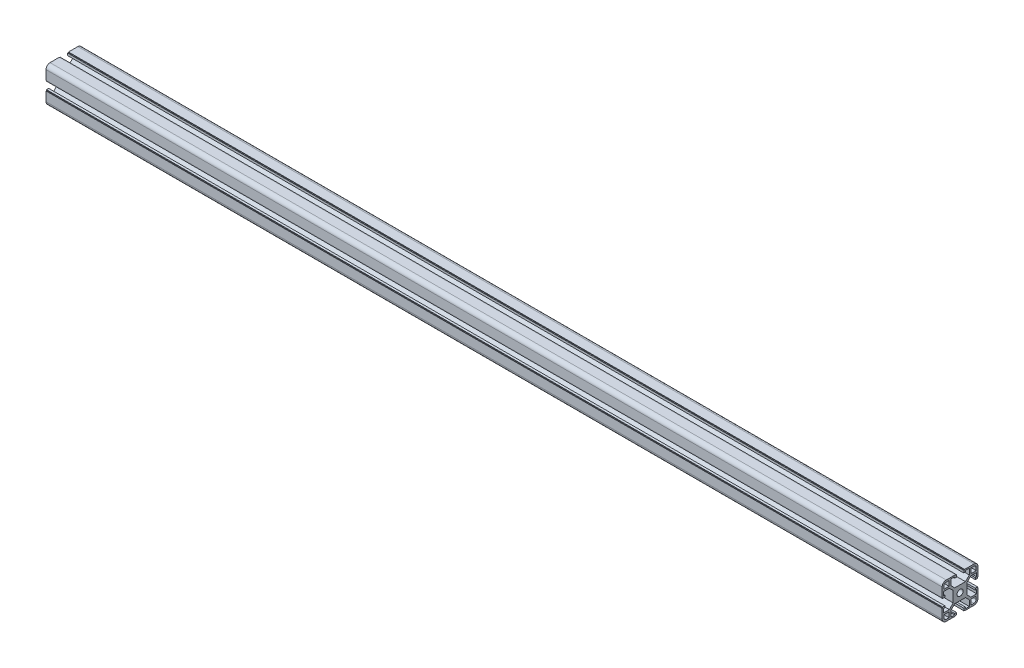
SolidWorks part; units mm, degrees
ref_plane "Front Plane" through (0, 0, 0) normal (0, 0, 1) x (1, 0, 0)
ref_plane "Top Plane" through (0, 0, 0) normal (0, 1, 0) x (1, 0, 0)
ref_plane "Right Plane" through (0, 0, 0) normal (1, 0, 0) x (0, 0, -1)
sketch "草图1" plane through (0, 0, 0) normal (0, 0, 1) x (1, 0, 0)
  line L0 (0, 0) -> (1000, 0)
  dimension "D1" = 1000
other "Aluminum profile 40 X 40B X R4.5(1)"
ref_plane "Plane1" through (0, 0, 0) normal (1, 0, 0) x (0, 1, 0)
sketch "Sketch1" plane through (0, 0, 0) normal (1, 0, 0) x (0, 1, 0)
  line L0 (-5.1, 20) -> (-5.1, 19.5)
  line L1 (-5.1, 19.5) -> (-4.1, 19.5)
  line L2 (-4.1, 19.5) -> (-4.1, 17)
  line L3 (-6.1, 18.5) -> (-10.3, 18.5)
  line L4 (-15.5, -20) -> (-5.1, -20)
  line L5 (-20, -15.5) -> (-20, -5.1)
  line L6 (15.5, 20) -> (5.1, 20)
  line L7 (20, 15.5) -> (20, 5.1)
  line L8 (0, 14.8756) -> (0, 0) construction
  line L9 (0, 0) -> (14.1675, 0) construction
  line L10 (-10.3, 18.5) -> (-10.3, 12)
  line L11 (-10.3, 12) -> (-6, 7.7)
  line L12 (-6, 7.7) -> (6, 7.7)
  line L13 (10.3, 12) -> (6, 7.7)
  line L14 (10.3, 18.5) -> (10.3, 12)
  line L15 (6.1, 18.5) -> (10.3, 18.5)
  line L16 (4.1, 19.5) -> (4.1, 17)
  line L17 (5.1, 19.5) -> (4.1, 19.5)
  line L18 (5.1, 20) -> (5.1, 19.5)
  line L19 (-5.1, 20) -> (-15.5, 20)
  line L20 (20, 5.1) -> (19.5, 5.1)
  line L21 (12.3, 18) -> (15.5, 18)
  line L22 (12.3, 18) -> (12.3, 12.3)
  line L23 (12.3, 12.3) -> (18, 12.3)
  line L24 (18, 15.5) -> (18, 12.3)
  line L25 (19.5, 5.1) -> (19.5, 4.1)
  line L26 (19.5, 4.1) -> (17, 4.1)
  line L27 (17, 6.1) -> (17, 4.1)
  line L28 (18.5, 6.1) -> (17, 6.1)
  line L29 (18.5, 6.1) -> (18.5, 10.3)
  line L30 (18.5, 10.3) -> (12, 10.3)
  line L31 (12, 10.3) -> (7.7, 6)
  line L32 (7.7, 6) -> (7.7, -6)
  line L33 (12, -10.3) -> (7.7, -6)
  line L34 (18.5, -10.3) -> (12, -10.3)
  line L35 (18.5, -6.1) -> (18.5, -10.3)
  line L36 (18.5, -6.1) -> (17, -6.1)
  line L37 (17, -4.1) -> (17, -6.1)
  line L38 (19.5, -4.1) -> (17, -4.1)
  line L39 (19.5, -5.1) -> (19.5, -4.1)
  line L40 (20, -5.1) -> (19.5, -5.1)
  line L41 (5.1, -20) -> (5.1, -19.5)
  line L42 (5.1, -19.5) -> (4.1, -19.5)
  line L43 (4.1, -19.5) -> (4.1, -17)
  line L44 (6.1, -17) -> (4.1, -17)
  line L45 (6.1, -18.5) -> (6.1, -17)
  line L46 (6.1, -18.5) -> (10.3, -18.5)
  line L47 (10.3, -18.5) -> (10.3, -12)
  line L48 (10.3, -12) -> (6, -7.7)
  line L49 (6, -7.7) -> (-6, -7.7)
  line L50 (-10.3, -12) -> (-6, -7.7)
  line L51 (-10.3, -18.5) -> (-10.3, -12)
  line L52 (-6.1, -18.5) -> (-10.3, -18.5)
  line L53 (-6.1, -18.5) -> (-6.1, -17)
  line L54 (-4.1, -17) -> (-6.1, -17)
  line L55 (-4.1, -19.5) -> (-4.1, -17)
  line L56 (-5.1, -19.5) -> (-4.1, -19.5)
  line L57 (-5.1, -20) -> (-5.1, -19.5)
  line L58 (-20, -5.1) -> (-19.5, -5.1)
  line L59 (5.1, -20) -> (15.5, -20)
  line L60 (-20, 5.1) -> (-20, 15.5)
  line L61 (-19.5, -5.1) -> (-19.5, -4.1)
  line L62 (-6.1, 18.5) -> (-6.1, 17)
  line L63 (-6.1, 17) -> (-4.1, 17)
  line L64 (6.1, 18.5) -> (6.1, 17)
  line L65 (4.1, 17) -> (6.1, 17)
  line L66 (-19.5, -4.1) -> (-17, -4.1)
  line L67 (-15.5, 18) -> (-12.3, 18)
  line L68 (-18, 15.5) -> (-18, 12.3)
  line L69 (-18, 12.3) -> (-12.3, 12.3)
  line L70 (-12.3, 18) -> (-12.3, 12.3)
  line L71 (-17, -6.1) -> (-17, -4.1)
  line L72 (-18.5, -6.1) -> (-17, -6.1)
  line L73 (-18.5, -6.1) -> (-18.5, -10.3)
  line L74 (-18.5, -10.3) -> (-12, -10.3)
  line L75 (-12, -10.3) -> (-7.7, -6)
  line L76 (-7.7, -6) -> (-7.7, 6)
  line L77 (-12, 10.3) -> (-7.7, 6)
  line L78 (-18.5, 10.3) -> (-12, 10.3)
  line L79 (-18.5, 6.1) -> (-18.5, 10.3)
  line L80 (-18.5, 6.1) -> (-17, 6.1)
  line L81 (-17, 4.1) -> (-17, 6.1)
  line L82 (-19.5, 4.1) -> (-17, 4.1)
  line L83 (-19.5, 5.1) -> (-19.5, 4.1)
  line L84 (-20, 5.1) -> (-19.5, 5.1)
  line L85 (20, -5.1) -> (20, -15.5)
  line L87 (-18, -12.3) -> (-12.3, -12.3)
  line L88 (-18, -12.3) -> (-18, -15.5)
  line L89 (-15.5, -18) -> (-12.3, -18)
  line L90 (-12.3, -12.3) -> (-12.3, -18)
  line L91 (12.3, -12.3) -> (18, -12.3)
  line L92 (12.3, -12.3) -> (12.3, -18)
  line L93 (12.3, -18) -> (15.5, -18)
  line L94 (18, -12.3) -> (18, -15.5)
  circle A0 centre (0, 0) radius 3.4
  arc A1 (-20, 15.5) -> (-15.5, 20) centre (-15.5, 15.5) cw
  arc A2 (20, 15.5) -> (15.5, 20) centre (15.5, 15.5) ccw
  arc A3 (-15.5, -20) -> (-20, -15.5) centre (-15.5, -15.5) cw
  arc A4 (15.5, -20) -> (20, -15.5) centre (15.5, -15.5) ccw
  arc A5 (-15.5, 18) -> (-18, 15.5) centre (-15.5, 15.5) ccw
  arc A6 (18, 15.5) -> (15.5, 18) centre (15.5, 15.5) ccw
  arc A7 (18, -15.5) -> (15.5, -18) centre (15.5, -15.5) cw
  arc A8 (-18, -15.5) -> (-15.5, -18) centre (-15.5, -15.5) ccw
  point P2 (0, 10)
  point P4 (0, 0)
  point P5 (-20, -20)
  point P6 (20, -20)
  point P7 (20, 20)
  point P8 (-20, 20)
  point P36 (-20, 20)
  point P39 (20, 20)
  point P121 (0, 0)
  dimension "D1" = 20.6
  dimension "D2" = 40
  dimension "D3" = 8.2
  dimension "D4" = 10.2
  dimension "D5" = 12.3
  dimension "D6" = 6.8
  dimension "D7" = 4.5
  dimension "D8" = 45
  dimension "D12" = 2
  dimension "D13" = 5.7
  dimension "D14" = 2
  dimension "D18" = 2.5
  dimension "D19" = 2.5
  dimension "D15" = 2.5
  dimension "D9" = 0.5
  dimension "D10" = 1.5
  dimension "D11" = 12
  dimension "D16" = 3
  dimension "D17" = 2
  dimension "D20" = 2
  dimension "D21" = 2
